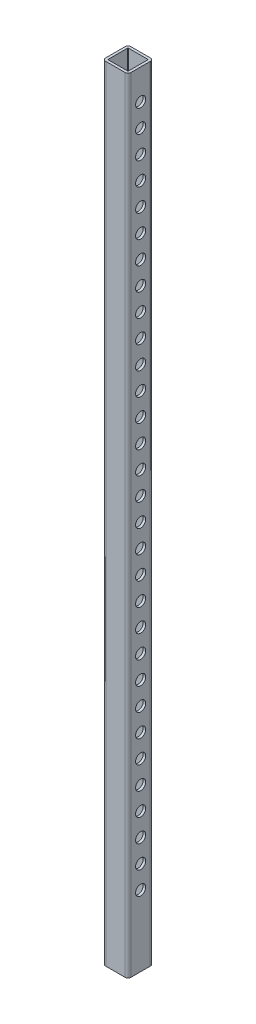
from build123d import *

# Parameters (mm, degrees)
EXTRUDE_1_DEPTH     = 1550
SKETCH_2_R          = 12
CUT_EXTRUDE_1_DEPTH = 10
SKETCH_3_R          = 16.065065839
SKETCH_3_R_2        = 15.441664685
EXTRUDE_2_DEPTH     = 5
SKETCH_4_W          = 38
SKETCH_4_H          = 630.491026123
EXTRUDE_3_DEPTH     = 5
SKETCH_5_R          = 10
CUT_EXTRUDE_2_DEPTH = 10


with BuildPart() as part:
    # 草图1 → 凸台-拉伸1 (new body)
    with BuildSketch(Plane(origin=(0, 0, 0), x_dir=(1, 0, 0), z_dir=(0, 1, 0))):
        with BuildLine():
            Line((-19, -12.278106509), (19, -12.278106509))
            ThreePointArc((19, -12.278106509), (23.242640687, -10.520747196), (25, -6.278106509))
            Line((25, -6.278106509), (25, 31.721893491))
            ThreePointArc((25, 31.721893491), (23.242640687, 35.964534178), (19, 37.721893491))
            Line((19, 37.721893491), (-19, 37.721893491))
            ThreePointArc((-19, 37.721893491), (-23.242640687, 35.964534178), (-25, 31.721893491))
            Line((-25, 31.721893491), (-25, -6.278106509))
            ThreePointArc((-25, -6.278106509), (-23.242640687, -10.520747196), (-19, -12.278106509))
        make_face()
        with BuildLine():
            Line((-19, -7.278106509), (19, -7.278106509))
            ThreePointArc((19, -7.278106509), (19.707106781, -6.98521329), (20, -6.278106509))
            Line((20, -6.278106509), (20, 31.721893491))
            ThreePointArc((20, 31.721893491), (19.707106781, 32.429000272), (19, 32.721893491))
            Line((19, 32.721893491), (-19, 32.721893491))
            ThreePointArc((-19, 32.721893491), (-19.707106781, 32.429000272), (-20, 31.721893491))
            Line((-20, 31.721893491), (-20, -6.278106509))
            ThreePointArc((-20, -6.278106509), (-19.707106781, -6.98521329), (-19, -7.278106509))
        make_face(mode=Mode.SUBTRACT)
    extrude(amount=EXTRUDE_1_DEPTH)

    # 草图2 → 切除-拉伸1 (cut)
    with BuildSketch(Plane(origin=(25, 0, 0), x_dir=(0, 0, -1), z_dir=(1, 0, 0))):
        with Locations((12.721893491, 1527.5)):
            Circle(SKETCH_2_R)
        with Locations((12.721893491, 1482.5)):
            Circle(SKETCH_2_R)
        with Locations((12.721893491, 1437.5)):
            Circle(SKETCH_2_R)
        with Locations((12.721893491, 1392.5)):
            Circle(SKETCH_2_R)
        with Locations((12.721893491, 1347.5)):
            Circle(SKETCH_2_R)
        with Locations((12.721893491, 1302.5)):
            Circle(SKETCH_2_R)
        with Locations((12.721893491, 1257.5)):
            Circle(SKETCH_2_R)
        with Locations((12.721893491, 1212.5)):
            Circle(SKETCH_2_R)
        with Locations((12.721893491, 1167.5)):
            Circle(SKETCH_2_R)
        with Locations((12.721893491, 1122.5)):
            Circle(SKETCH_2_R)
        with Locations((12.721893491, 1077.5)):
            Circle(SKETCH_2_R)
        with Locations((12.721893491, 1032.5)):
            Circle(SKETCH_2_R)
        with Locations((12.721893491, 987.5)):
            Circle(SKETCH_2_R)
        with Locations((12.721893491, 942.5)):
            Circle(SKETCH_2_R)
        with Locations((12.721893491, 897.5)):
            Circle(SKETCH_2_R)
    extrude(amount=-CUT_EXTRUDE_1_DEPTH, mode=Mode.SUBTRACT)

    # 草图3 → 凸台-拉伸2 (add)
    with BuildSketch(Plane(origin=(25, 0, 0), x_dir=(0, 0, -1), z_dir=(1, 0, 0))):
        with Locations((12.721893491, 897.5)):
            Circle(SKETCH_3_R)
        with Locations((12.721893491, 1527.5)):
            Circle(SKETCH_3_R_2)
    extrude(amount=-EXTRUDE_2_DEPTH)

    # 草图4 → 凸台-拉伸3 (add)
    with BuildSketch(Plane(origin=(25, 0, 0), x_dir=(0, 0, -1), z_dir=(1, 0, 0))):
        with Locations((12.721893491, 1196.647134408)):
            Rectangle(SKETCH_4_W, SKETCH_4_H)
    extrude(amount=-EXTRUDE_3_DEPTH)

    # 草图5 → 切除-拉伸2 (cut)
    with BuildSketch(Plane(origin=(25, 0, 0), x_dir=(0, 0, -1), z_dir=(1, 0, 0))):
        with Locations((12.721893491, 1490)):
            Circle(SKETCH_5_R)
        with Locations((12.721893491, 1445)):
            Circle(SKETCH_5_R)
        with Locations((12.721893491, 1400)):
            Circle(SKETCH_5_R)
        with Locations((12.721893491, 1355)):
            Circle(SKETCH_5_R)
        with Locations((12.721893491, 1310)):
            Circle(SKETCH_5_R)
        with Locations((12.721893491, 1265)):
            Circle(SKETCH_5_R)
        with Locations((12.721893491, 1220)):
            Circle(SKETCH_5_R)
        with Locations((12.721893491, 1175)):
            Circle(SKETCH_5_R)
        with Locations((12.721893491, 1130)):
            Circle(SKETCH_5_R)
        with Locations((12.721893491, 1085)):
            Circle(SKETCH_5_R)
        with Locations((12.721893491, 1040)):
            Circle(SKETCH_5_R)
        with Locations((12.721893491, 995)):
            Circle(SKETCH_5_R)
        with Locations((12.721893491, 950)):
            Circle(SKETCH_5_R)
        with Locations((12.721893491, 905)):
            Circle(SKETCH_5_R)
        with Locations((12.721893491, 860)):
            Circle(SKETCH_5_R)
        with Locations((12.721893491, 815)):
            Circle(SKETCH_5_R)
        with Locations((12.721893491, 770)):
            Circle(SKETCH_5_R)
        with Locations((12.721893491, 725)):
            Circle(SKETCH_5_R)
        with Locations((12.721893491, 680)):
            Circle(SKETCH_5_R)
        with Locations((12.721893491, 635)):
            Circle(SKETCH_5_R)
        with Locations((12.721893491, 590)):
            Circle(SKETCH_5_R)
        with Locations((12.721893491, 545)):
            Circle(SKETCH_5_R)
        with Locations((12.721893491, 500)):
            Circle(SKETCH_5_R)
        with Locations((12.721893491, 455)):
            Circle(SKETCH_5_R)
        with Locations((12.721893491, 410)):
            Circle(SKETCH_5_R)
        with Locations((12.721893491, 365)):
            Circle(SKETCH_5_R)
        with Locations((12.721893491, 320)):
            Circle(SKETCH_5_R)
        with Locations((12.721893491, 275)):
            Circle(SKETCH_5_R)
        with Locations((12.721893491, 230)):
            Circle(SKETCH_5_R)
        with Locations((12.721893491, 185)):
            Circle(SKETCH_5_R)
        with Locations((12.721893491, 140)):
            Circle(SKETCH_5_R)
    extrude(amount=-CUT_EXTRUDE_2_DEPTH, mode=Mode.SUBTRACT)


solid = part.part
